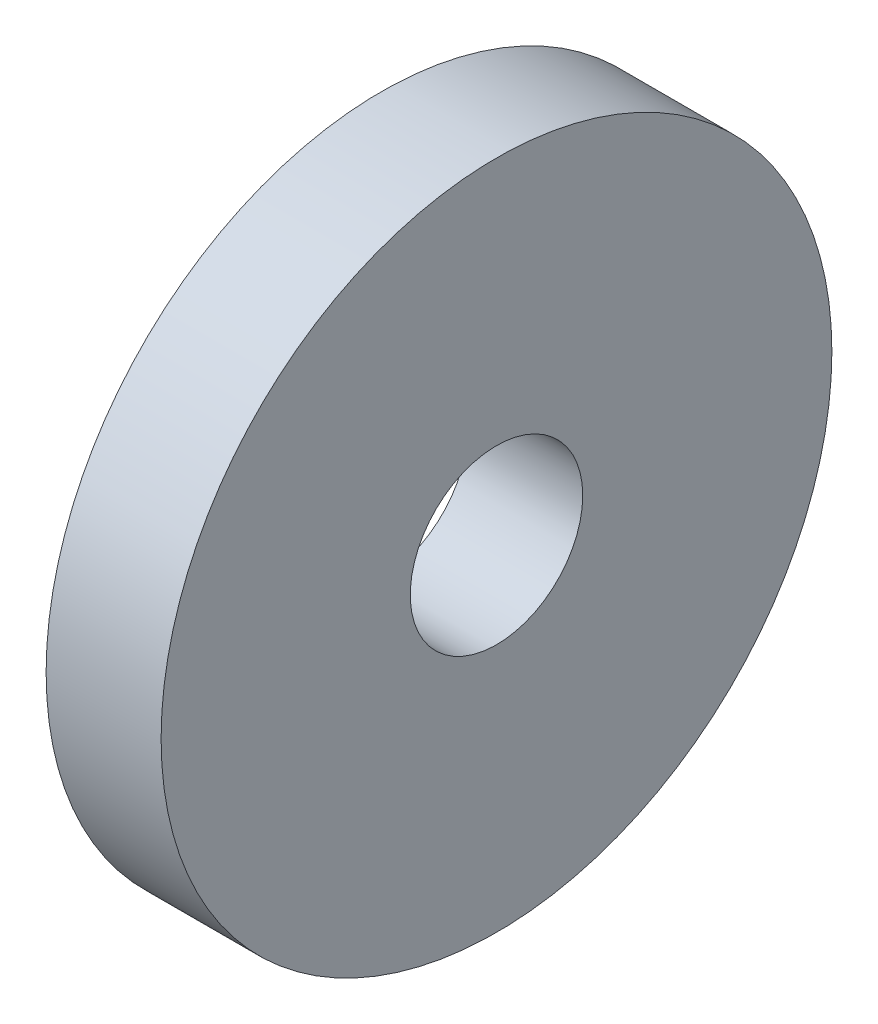
SolidWorks part; units mm, degrees
ref_plane "前视基准面" through (0, 0, 0) normal (0, 0, 1) x (1, 0, 0)
ref_plane "上视基准面" through (0, 0, 0) normal (0, 1, 0) x (1, 0, 0)
ref_plane "右视基准面" through (0, 0, 0) normal (1, 0, 0) x (0, 0, -1)
sketch "草图1" plane through (0, 0, 0) normal (1, 0, 0) x (0, 0, -1)
  circle A0 centre (0, 0) radius 17.5
  circle A1 centre (0, 0) radius 4.5
  dimension "D1" = 35
  dimension "D2" = 9
extrude "凸台-拉伸1" add sketch "草图1" along normal blind 6
